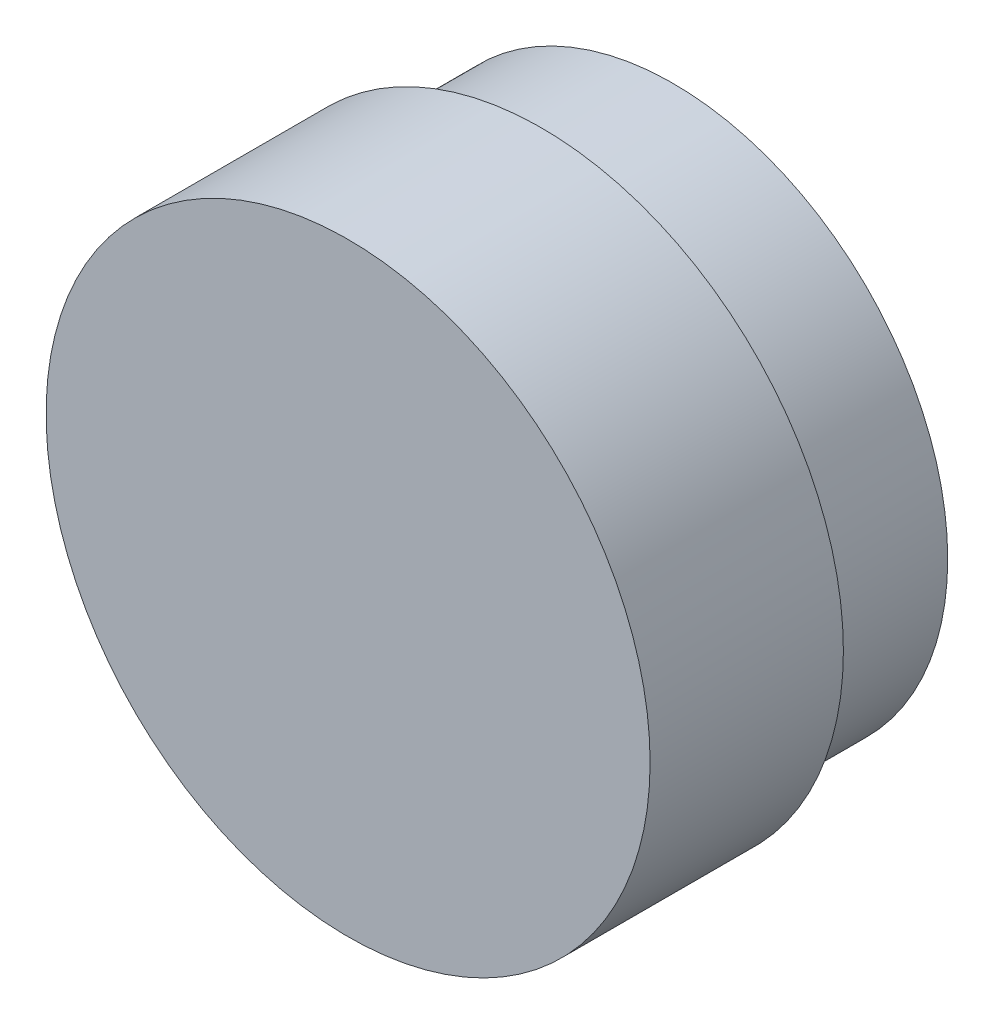
SolidWorks part; units mm, degrees
material "普通碳钢"
ref_plane "Front Plane" through (0, 0, 0) normal (0, 0, 1) x (1, 0, 0)
ref_plane "Top Plane" through (0, 0, 0) normal (0, 1, 0) x (1, 0, 0)
ref_plane "Right Plane" through (0, 0, 0) normal (1, 0, 0) x (0, 0, -1)
sketch "Sketch1" plane through (0, 0, 0) normal (0, 0, 1) x (1, 0, 0)
  circle A0 centre (0, 0) radius 25
  dimension "D1" = 50
extrude "Boss-Extrude1" add sketch "Sketch1" along normal blind 12
sketch "Sketch2" plane through (0, 0, 12) normal (0, 0, 1) x (1, 0, 0)
  circle A0 centre (0, 0) radius 27.5
  dimension "D1" = 55
extrude "Boss-Extrude2" add sketch "Sketch2" along normal blind 17.6
